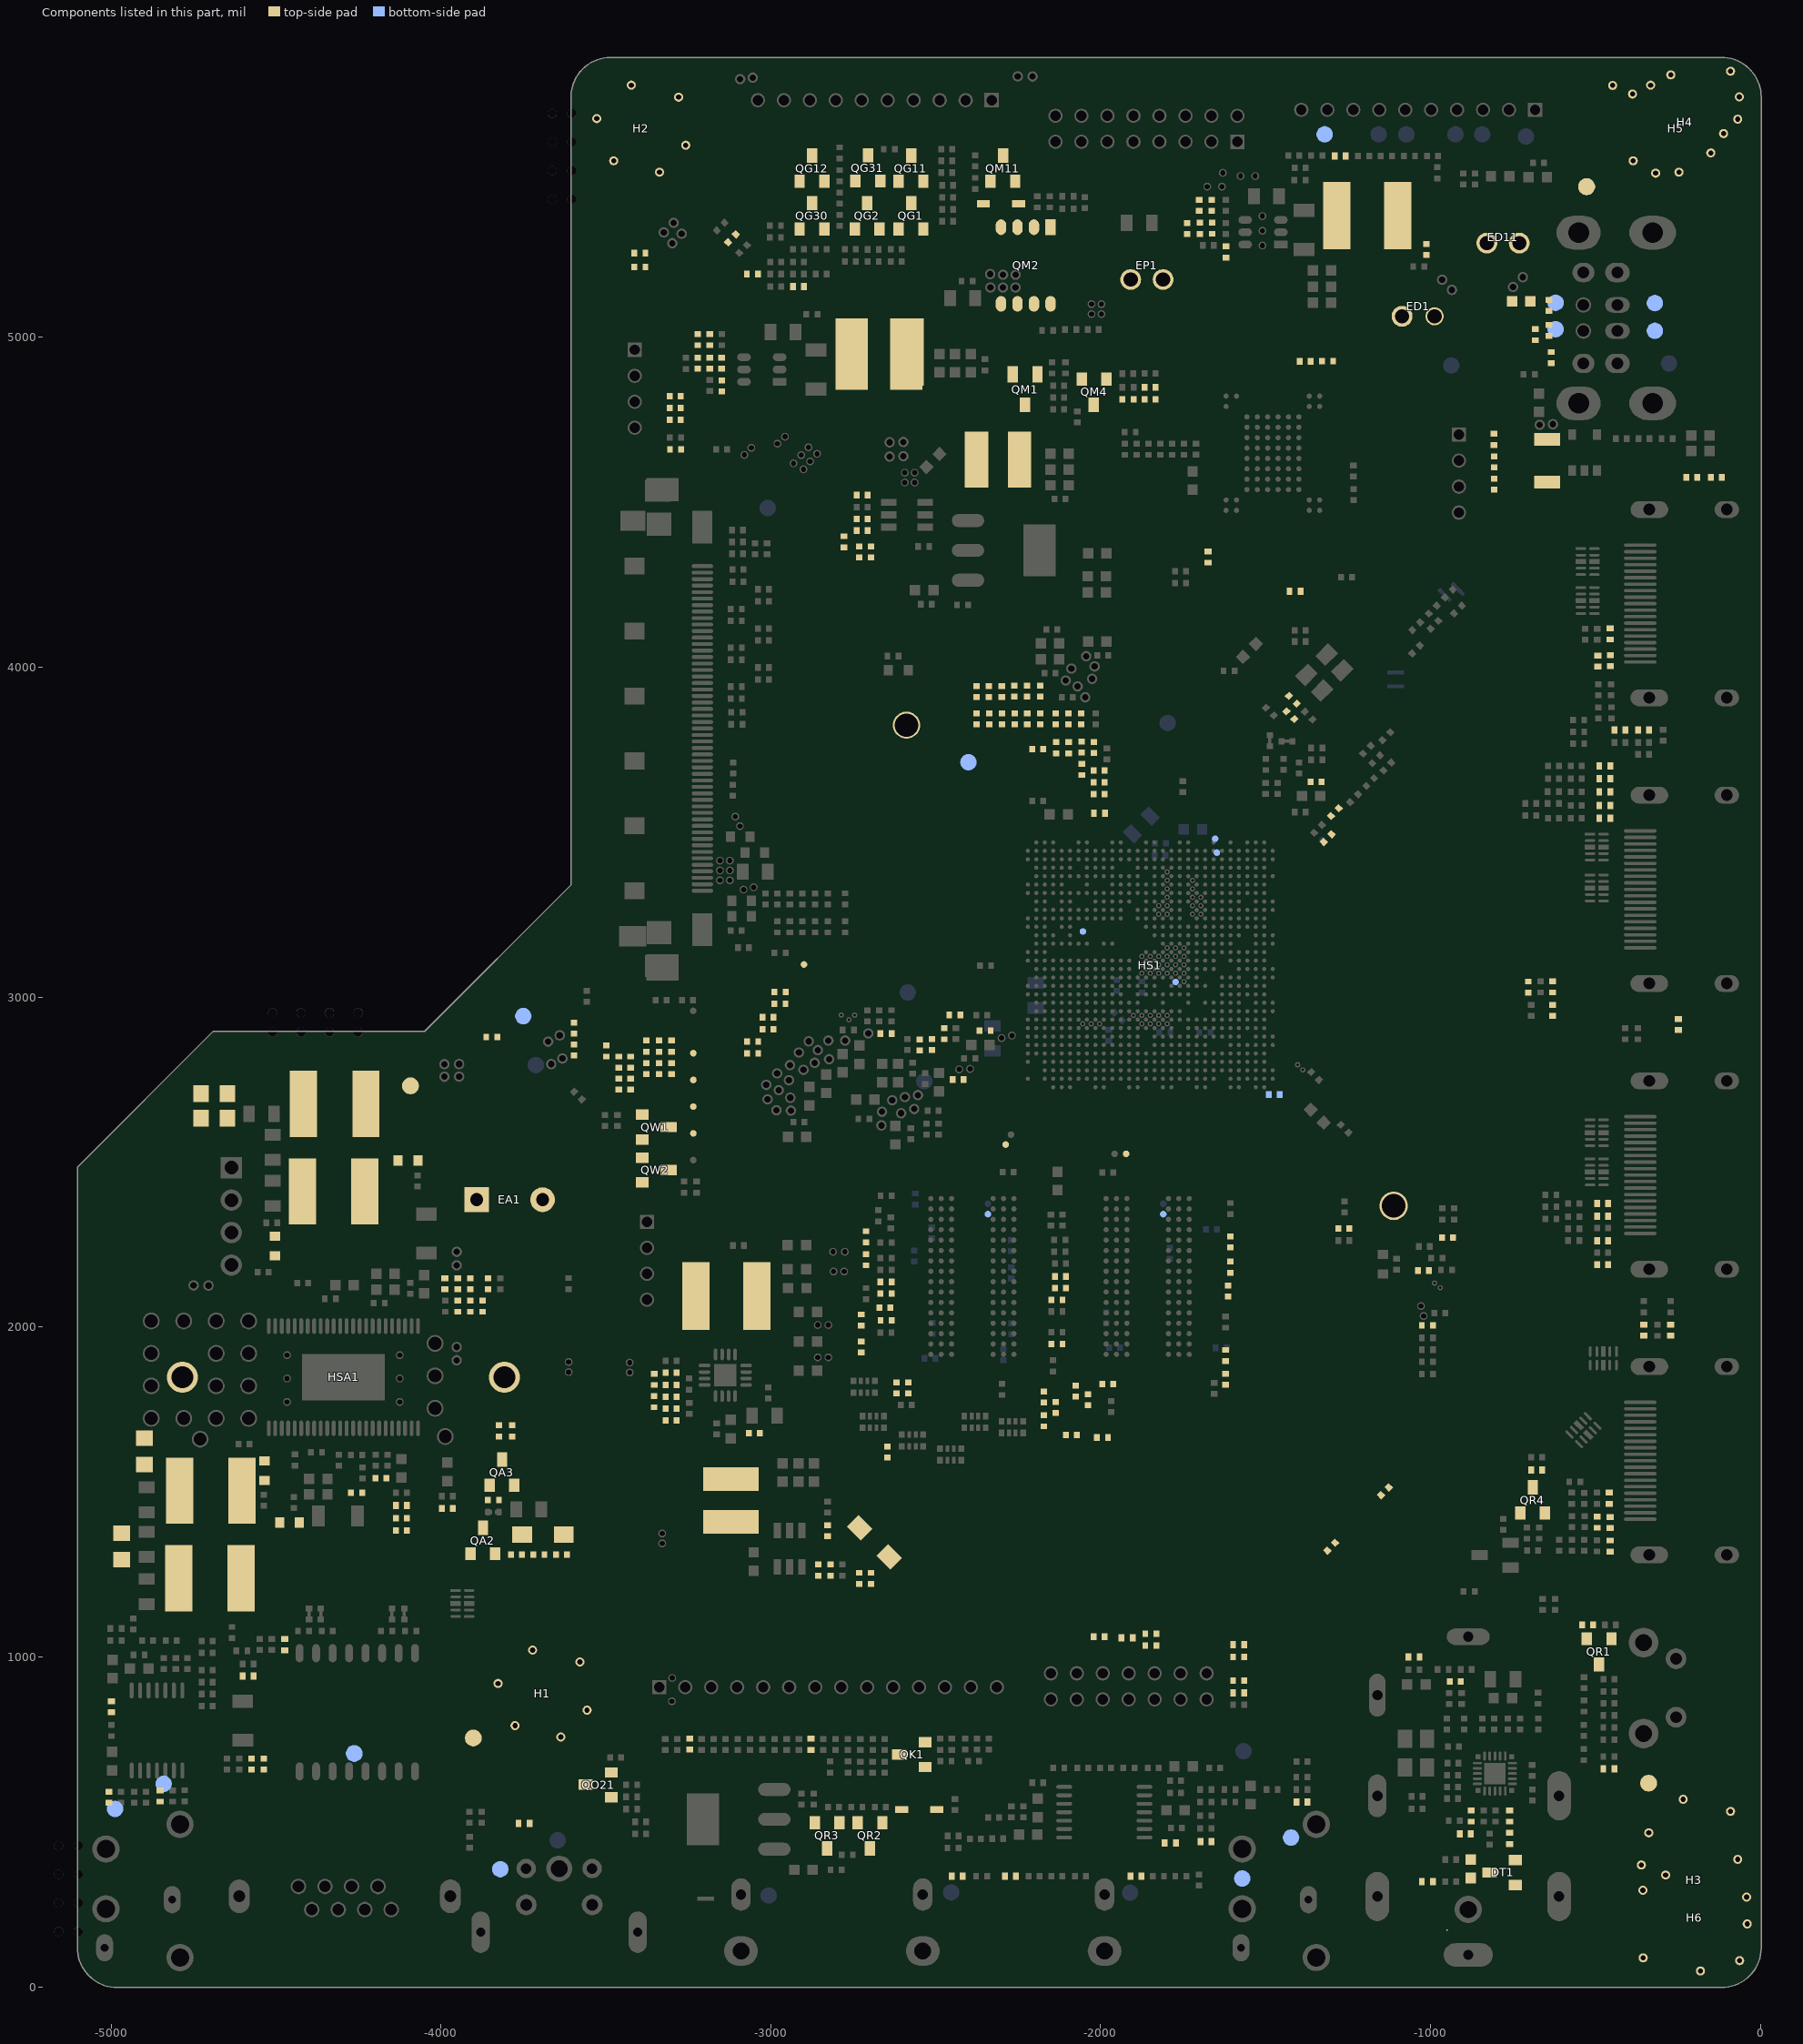
[diagram p0: the components of this part, seen from the top]
# Altium PCB MISC86290.PcbDoc (part 3 of 31)
Units mil, origin at the board's own origin, x right, y up, seen from the top; angles counter-clockwise.
Board outline 5104.71 x 5851.49 mil, 2 copper layers (TopLayer, BottomLayer), stack 61.855 mil thick; 1026 components, 667 nets, 4280 pads, 2294 vias.

## Components (designator, comment, footprint, x,y, rotation, side; value= is the part's Value field where it differs from the comment) (continued)
D41 "NC/SFI0402-240E-2R5PP-LF" DIODE-S0402 -630,2960 r90 top
DA1 "NC/AVLC18S02003" DIODE-S0402 -1582,891 r0 top
DA2 "NC/AVLC18S02003" DIODE-S0402 -1582,1037 r180 top
DA5 "NC/AVLC18S02003" DIODE-S0402 -1920,1058 r0 top
DA6 "NC/AVLC18S02003" DIODE-S0402 -2005,1061 r180 top
DA9 "Switching diode,DIO SW S,200mA,75V,MiniMELF,SMD,LL4148,FORMOSA" DIODE-S0805 -3691,1371 r180 top
DBS7 "DOLBY PLUS" "DOLBY PLUS-SILK" -1080.5,2556.5 r90 bottom
DD2 "Zener diode,DIO ZEN,5.6V,500mW,SOD-80,SMD,BZV55C5V6,GOOD-ARK" DIODE-S0805 -2686,1347 r315 top
DE1 "NC/AIES12U020R2" DIODE-S0402 -4584.6,941.4 r0 top
DE2 "NC/AIES12U020R2" DIODE-S0402 -4473.96,1036.98 r270 top
DF5 "NC/NC/AIES12U020R2" DIODE-S0402 -641.25,5021.27 r90 top
DF6 "NC/NC/AIES12U020R2" DIODE-S0402 -641.25,5096.73 r270 top
DG1 "NC/SFI0402-240E-2R5PP-LF" DIODE-S0402 -2916,5154 r180 top
DG11 "NC/SFI0402-240E-2R5PP-LF" DIODE-S0402 -3056,5192 r0 top
DH1 "NC/TVS diode,DIO ESD,0.5pF,25V,0402 DFN,SMD,AZ5325-01F.R7G,Amazing" DIODE-S0402 -354,3810 r180 top
DH2 "NC/TVS diode,DIO ESD,0.5pF,25V,0402 DFN,SMD,AZ5325-01F.R7G,Amazing" DIODE-S0402 -426,3810 r180 top
DH3 "NC/TVS diode,DIO ESD,0.5pF,25V,0402 DFN,SMD,AZ5325-01F.R7G,Amazing" DIODE-S0402 -455,4019.73 r90 top
DH4 "NC/TVS diode,DIO ESD,0.5pF,25V,0402 DFN,SMD,AZ5325-01F.R7G,Amazing" DIODE-S0402 -493,4019 r90 top
DH5 "NC/TVS diode,DIO ESD,0.5pF,25V,0402 DFN,SMD,AZ5325-01F.R7G,Amazing" DIODE-S0402 -456,4101 r90 top
DH11 "NC/TVS diode,DIO ESD,0.5pF,25V,0402 DFN,SMD,AZ5325-01F.R7G,Amazing" DIODE-S0402 -472,3701 r0 top
DH12 "NC/TVS diode,DIO ESD,0.5pF,25V,0402 DFN,SMD,AZ5325-01F.R7G,Amazing" DIODE-S0402 -472,3662 r0 top
DH13 "NC/TVS diode,DIO ESD,0.5pF,25V,0402 DFN,SMD,AZ5325-01F.R7G,Amazing" DIODE-S0402 -472,3622 r0 top
DH14 "NC/TVS diode,DIO ESD,0.5pF,25V,0402 DFN,SMD,AZ5325-01F.R7G,Amazing" DIODE-S0402 -472,3581 r0 top
DH15 "NC/TVS diode,DIO ESD,0.5pF,25V,0402 DFN,SMD,AZ5325-01F.R7G,Amazing" DIODE-S0402 -472,3542 r0 top
DH21 "NC/TVS diode,DIO ESD,0.5pF,25V,0402 DFN,SMD,AZ5325-01F.R7G,Amazing" DIODE-S0402 -478,2189 r0 top
DH22 "NC/TVS diode,DIO ESD,0.5pF,25V,0402 DFN,SMD,AZ5325-01F.R7G,Amazing" DIODE-S0402 -478,2261 r0 top
DH23 "NC/TVS diode,DIO ESD,0.5pF,25V,0402 DFN,SMD,AZ5325-01F.R7G,Amazing" DIODE-S0402 -478,2336 r0 top
DH24 "NC/TVS diode,DIO ESD,0.5pF,25V,0402 DFN,SMD,AZ5325-01F.R7G,Amazing" DIODE-S0402 -478,2374 r0 top
DH31 "NC/TVS diode,DIO ESD,0.5pF,25V,0402 DFN,SMD,AZ5325-01F.R7G,Amazing" DIODE-S0402 -456,1407 r270 top
DH32 "NC/TVS diode,DIO ESD,0.5pF,25V,0402 DFN,SMD,AZ5325-01F.R7G,Amazing" DIODE-S0402 -456,1336 r270 top
DH33 "NC/TVS diode,DIO ESD,0.5pF,25V,0402 DFN,SMD,AZ5325-01F.R7G,Amazing" DIODE-S0402 -495,1408 r90 top
DH34 "NC/TVS diode,DIO ESD,0.5pF,25V,0402 DFN,SMD,AZ5325-01F.R7G,Amazing" DIODE-S0402 -458,1481 r90 top
DH35 "NC/TVS diode,DIO ESD,0.5pF,25V,0402 DFN,SMD,AZ5325-01F.R7G,Amazing" DIODE-S0402 -353.27,1990.5 r90 top
DH36 "NC/TVS diode,DIO ESD,0.5pF,25V,0402 DFN,SMD,AZ5325-01F.R7G,Amazing" DIODE-S0402 -272,1990.5 r90 top
DH37 "NC/TVS diode,DIO ESD,0.5pF,25V,0402 DFN,SMD,AZ5325-01F.R7G,Amazing" DIODE-S0402 -248.64,2917.23 r270 top
DI1 "NC/TVS diode,DIO ESD,3pF,58V,0402,SMD,SDV1005H260C030YPTF,Sunlord" DIODE-S0402 -2435,335 r0 top
DI2 "NC/TVS diode,DIO ESD,3pF,58V,0402,SMD,SDV1005H260C030YPTF,Sunlord" DIODE-S0402 -2274,335 r0 top
DI3 "NC/TVS diode,DIO ESD,3pF,58V,0402,SMD,SDV1005H260C030YPTF,Sunlord" DIODE-S0402 -1893,335 r180 top
DK9 "NC/AVLC18S02003" DIODE-S0402 -2878.25,735 r270 top
DK10 "NC/AVLC18S02003" DIODE-S0402 -3245.92,735.99 r270 top
DM0 "TEST" TP -320,5020 r180 bottom
DM1 "TEST" TP -620.95,5024.72 r180 bottom
DM11 "NC/Switching diode,DIO SW S,150mA,75V,SOD-323,SMD,1N4148WS,BLUE ROCKET" DIODE-S-12 -2302.25,5405 r180 top
DO1 "NC/SFI0402-240E-2R5PP-LF" DIODE-S0402 -3748.25,495 r180 top
DO2 "NC/SFI0402-240E-2R5PP-LF" DIODE-S0402 -1022,2171 r0 top
DO11 "NC/NC?" DIODE-S0402 -1390,559.5 r0 top
DO12 "NC/NC?" DIODE-S0402 -1681,440 r0 top
DO31 "NC/NC?" DIODE-S0402 -4851.5,578 r270 top
DO32 "NC/NC?" DIODE-S0402 -5006.75,573.94 r270 top
DP0 "TEST" TP -320,5104 r180 bottom
DP1 "TEST" TP -620.95,5105.12 r180 bottom
DQS0 "TEST" TP-20#1 -1923,2525 r90 top
DQS0# "TEST" TP-20#1 -1958,2525 r90 top
DQS1 "TEST" TP-20#1 -1810.35,2342.13 r90 bottom
DQS1# "TEST" TP-20#1 -1810.35,2373.62 r90 bottom
DQS2 "TEST" TP-20#1 -2288,2553 r90 top
DQS2# "TEST" TP-20#1 -2272,2583 r90 top
DQS3 "TEST" TP-20#1 -2341.85,2342.13 r90 bottom
DQS3# "TEST" TP-20#1 -2341.85,2373.62 r90 bottom
DR1 "NC/TVS diode,DIO ESD,3pF,58V,0402,SMD,SDV1005H260C030YPTF,Sunlord" DIODE-S0402 -678.5,1566.5 r0 top
DR2 "TVS diode,DIO ESD,3pF,58V,0402,SMD,SDV1005H260C030YPTF,Sunlord" DIODE-S0402 -459.5,660.5 r0 top
DR3 "Switching diode,DIO SW S,150mA,75V,SOD-323,SMD,1N4148WS,BLUE ROCKET" DIODE-S-12 -2550,537 r180 top
DR4 "NC/TVS diode,DIO ESD,3pF,58V,0402,SMD,SDV1005H260C030YPTF,Sunlord" DIODE-S0402 -1474,2704.5 r180 bottom
DR5 "NC/TVS diode,DIO ESD,3pF,58V,0402,SMD,SDV1005H260C030YPTF,Sunlord" DIODE-S0402 -2004,3557.11 r180 top
DT1 "Switching diode,DIO SW D2,75V,SOT-23,SMD,KAV99,KEXIN" SO-23 -782.86,346.15 r270 top
DT2 "NC/TVS diode,DIO ESD,3pF,58V,0402,SMD,SDV1005H260C030YPTF,Sunlord" DIODE-S0402 -208,4576 r0 top
DT3 "NC/TVS diode,DIO ESD,3pF,58V,0402,SMD,SDV1005H260C030YPTF,Sunlord" DIODE-S0402 -134,4576 r180 top
DU1 "NC/AIES12U020R2" DIODE-S0402 -634,4939 r90 top
DU2 "NC/AIES12U020R2" DIODE-S0402 -682.3,5008.37 r270 top
DVDD_DDR "TEST" TP-20#1 -1773,3046.11 r90 bottom
DW1 "NC/AIES12U020R2" DIODE-S0402 -1274,5550 r180 top
DW2 "NC/AIES12U020R2" DIODE-S0402 -1411,4230 r0 top
EA1 "Aluminium electrolytic capacitor,CAP AL,16V,470uF,±20%,KM,P,5.0mm,10×12.5,DIP,TP,Samxon" EC(10*13)-V-5.0-1 -3792,2386 r0 top
ED1 "Aluminium electrolytic capacitor,CAP AL,10V,470uF,±20%,PKZH,P,2.5mm,6.3×11,DIP,TP,Koshin" EC(6.3*11)-V-2.5#1 -1037.21,5064 r0 top
ED11 "Aluminium electrolytic capacitor,CAP AL,10V,470uF,±20%,PKZH,P,2.5mm,6.3×11,DIP,TP,Koshin" EC(6.3*11)-V-2.5#2 -780.27,5286 r0 top
EJ_TCK "TEST" TP-20#1 -3235,2587 r0 top
EJ_TDI "TEST" TP-20#1 -3235,2668 r0 top
EJ_TDO "TEST" TP-20#1 -3235,2749 r0 top
EJ_TMS "TEST" TP-20#1 -3235,2830 r0 top
EP1 "Aluminium electrolytic capacitor,CAP AL,16V,220uF,±20%,LD,KF,P,2.5mm,6.3×11,DIP,TP,CapXon" EC(6.3*11)-V-2.5#3 -1860,5175.5 r0 top
FT1 "Ferrite bead,BEAD,120ohm,0402,500mA,SMD,TP,GZ1005U121CTF,Sunlord" L0402 -1050,1000 r0 top
FU1 "NC/Resettable fuse,FUSE PTC,1.1A,6V,1206,SMD,TP,TLC" FUSE1.1A-S -647,4626 r270 top
H1 "Location hole" ASSE3.5C-3#1 -3685.04,885.83 r0 top locked
H2 "Location hole" ASSE3.5C-3#2 -3385.83,5629.92 r0 top locked
H3 "Location hole" ASSE3.5C-3#3 -196.85,433.07 r0 top locked
H4 "Location hole" ASSE3.5C-3#4 -196.85,5708.66 r0 top locked
H5 "Location hole" ASSE3.5C-3#5 -295.28,5629.92 r0 top locked
H6 "Location hole" ASSE5.0C-3 -196.85,196.85 r0 top locked
HOST_WAKE_WL "TEST" TP -1321.08,5615.53 r180 bottom locked
HP_DET "TEST" TP -3750.5,2942.5 r180 bottom
HP_OUT_L "TEST" TP -1570.87,328 r90 bottom
HP_OUT_R "TEST" TP -1423,452 r90 bottom
HS1 "Heat sink,AL6063-T5,55.0×55.0×10.0mm,black,anodized,fin type,LHD" HS(55*55*10) -1849.72,3098.03 r270 top locked
HSA1 "NC/Heat sink,27.5×10.0×10.0mm,AL6063-T5,black,anodized,fin type,WT" HS(27*10*10)-1 -4295.75,1847.75 r90 top locked
I2S_IN_MCK "TEST" TP-20#1 -2899.5,3099 r90 top
LA1 "Power inductor,Power Inductor,15uH,±20%,2.10A,DR6.0×4.5,SMD,MPIT6045-150M-LF,Microgate" L(6.0*4.5)-S#1 -4700.74,1238 r180 top
LA2 "Power inductor,Power Inductor,15uH,±20%,2.10A,DR6.0×4.5,SMD,MPIT6045-150M-LF,Microgate" L(6.0*4.5)-S#1 -4697.39,1503.52 r180 top
LA3 "Power inductor,Power Inductor,15uH,±20%,2.10A,DR6.0×4.5,SMD,MPIT6045-150M-LF,Microgate" L(6.0*4.5)-S#1 -4325,2411 r0 top
LA4 "Power inductor,Power Inductor,15uH,±20%,2.10A,DR6.0×4.5,SMD,MPIT6045-150M-LF,Microgate" L(6.0*4.5)-S#1 -4322,2676.38 r180 top
LA10 "0ohm-0402-±5%-1/16W" L0402 -3988,2131 r270 top
LA12 "0ohm-0402-±5%-1/16W" L0402 -4120,1459 r0 top
LD1 "NC/Power inductor,Power Inductor,4.7uH,±20%,3.3A,DR6.0×4.5,SMD,SWPA6045S4R7MT,Sunlord" L(6.0*4.5)-S#2 -1192.25,5369 r0 top
LD2 "Power inductor,Power Inductor,4.7uH,±20%,2.8A,0.32×1P,DR5.8×4.5,SMD,PIO54-4R7MTP02,FH" L(5.8*4.5)-S -2672.12,4949.21 r0 top
LD3 "NC/Power inductor,Power Inductor,4.7uH,±20%,3.8A,DR6.0×4.5,SMD,MPIT6045-4R7M-LF,Microgate" L(6.0*4.5)-S#2 -2670,4955.5 r0 top
LD4 "Power inductor,Power Inductor,4.7uH,±20%,3.3A,DR6.0×4.5,SMD,PRS6045-4R7MTP02,FH" L(6.0*4.5)-S#2 -1192.25,5369 r0 top
LD21 "Power inductor,Power Inductor,2.2uH,±20%,2A,0.28×1P,DR4.5×3.2,SMD,PIO43-2R2MTP02,FH" L(4.5*3.5)-S -3121,1474 r90 top
LD31 "Power inductor,Power Inductor,2.2μH,±30%,4.6A,6045,SMT,PRS6045-2R2NTP02,FH" L(6.0*4.5)-S#2 -3134.25,2094 r0 top
LD51 "Power inductor,Power Inductor,2.2uH,±20%,2A,0.28×1P,DR4.5×3.2,SMD,PIO43-2R2MTP02,FH" L(4.5*3.5)-S -2311.2,4629.43 r0 top
LF1 "0ohm-0402-±5%-1/16W" L0402 -1675,4334 r270 top
LINEOUT_L "TEST" TP -4988,539 r90 bottom
LINEOUT_R "TEST" TP -4840.5,615 r90 bottom
LO1 "0ohm-0402-±5%-1/16W" R0402 -1347.27,3653 r0 top
LO2 "Ferrite bead,BEAD,120ohm,0402,500mA,SMD,TP,GZ1005U121CTF,Sunlord" L0402 -1789,436 r180 top
LO3 "Ferrite bead,BEAD,120ohm,0402,500mA,SMD,TP,GZ1005U121CTF,Sunlord" L0402 -4999,849 r90 top
LT3 "0ohm-0402-±5%-1/16W" L0402 -894.9,463.14 r180 top
LT4 "SDCL1005CR33JTDF" L0402 -1009.7,318.3 r180 top
LT5 "SDCL1005CR33JTDF" L0402 -876.89,517.36 r270 top
LT6 "SDCL1005CR33JTDF" L0402 -759.9,517.37 r270 top
LT7 "0ohm-0402-±5%-1/16W" L0402 -760.22,449.51 r270 top
LT9 "NC/Multilayer inductor,HF Inductor,180nH,±5%,0603,SMD,SDCL1608CR18JTDF,Sunlord" L0603 -877.7,357.3 r90 top
LT10 "NC/" R0402 -924.82,925.61 r0 top
LU11 "HCB1608KF-121T20(120ohm-2000mA)" L0603 -725,5110 r0 top
M1 "MARK" MARK -3902,754 r0 top
M2 "MARK" MARK -527,5457 r0 top
M3 "MARK" MARK -339,617 r0 top
M4 "MARK" MARK -4092.5,2731 r0 top
M5 "MARK" MARK -527,5457 r180 bottom
M6 "MARK" MARK -4263,707 r180 bottom
MAC "MAC" Barcode -2576,4726 r180 bottom
Manufacture_Info "Manufacture_Info" Manufacture_Info -1486,4578 r270 top
MCP_TEST "TEST" TP-20#1 -2054,3199 r180 bottom
MOD_1V2 "TEST" TP -2401,3712.11 r90 bottom
NC/ESD "NC/ESD" ESD -926.56,194.83 r225 top
OPTICAL "TEST" TP -3820.25,356.18 r90 bottom
P1(用于U1上) "Thermal grease,0.05g,Other,white,NULL" PCB_TIME -386,-235 r180 top
PM_RX "TEST" TP-20#2 -1648,3438 r180 bottom
PM_TX "TEST" TP-20#2 -1653,3480 r180 bottom
QA2 "General-purpose transistor,Dynatron,PNP,0.2A,40V,30-100,SOT-23,MMBT3906-(100-300),BLUE ROCKET" SOT-23 -3873,1353 r180 top
QA3 "General-purpose transistor,Dynatron,NPN,0.2A,40V,30-300,SOT-23,MMBT3904(f≥350MHz),BLUE ROCKET" SOT-23 -3815,1560 r180 top
QG1 "NC/General-purpose transistor,Dynatron,NPN,0.2A,40V,60-300,SOT-23,KMBT3904,KEXIN" SOT-23 -2575.25,5369 r180 top
QG2 "NC/General-purpose transistor,Dynatron,NPN,0.2A,40V,60-300,SOT-23,KMBT3904,KEXIN" SOT-23 -2708,5369 r180 top
QG11 "NC/General-purpose transistor,Dynatron,NPN,0.2A,40V,60-300,SOT-23,KMBT3904,KEXIN" SOT-23 -2575.25,5513.12 r180 top
QG12 "NC/General-purpose transistor,Dynatron,NPN,0.2A,40V,60-300,SOT-23,KMBT3904,KEXIN" SOT-23 -2875.31,5513.12 r180 top
QG30 "NC/General-purpose transistor,Dynatron,NPN,0.2A,40V,60-300,SOT-23,KMBT3904,KEXIN" SOT-23 -2875.31,5369 r180 top
QG31 "NC/General-purpose transistor,Dynatron,NPN,0.2A,40V,60-300,SOT-23,KMBT3904,KEXIN" SOT-23 -2706,5514 r180 top
QK1 "General-purpose transistor,Dynatron,NPN,0.2A,40V,60-300,SOT-23,KMBT3904,KEXIN" SOT-23 -2572.5,703.5 r270 top
QM1 "MOSFET,PMOS,-4.2A,-30V,0.052ohm@ID=-4.2A@VGS=-10V,SOT23-3,AO3401,BLUE ROCKET" SOT-23-1 -2229,4841 r0 top
QM2 "MOSFET,PMOS,-5.7A,-30V,0.07ohm@ID=-4.4A@VGS=-4.5V,SOP-8,KO4459,KEXIN" SO-8 -2227.25,5218 r270 top locked
QM4 "General-purpose transistor,Dynatron,NPN,0.2A,40V,60-300,SOT-23,KMBT3904,KEXIN" SOT-23 -2020.25,4834 r0 top
QM11 "General-purpose transistor,Dynatron,NPN,0.2A,40V,60-300,SOT-23,KMBT3904,KEXIN" SOT-23 -2296.75,5513.13 r180 top
QO21 "General-purpose transistor,Dynatron,NPN,0.2A,40V,60-300,SOT-23,KMBT3904,KEXIN" SOT-23 -3523.5,612 r270 top
QR1 "KMBT3906" SOT-23 -489,1015 r0 top
QR2 "KMBT3906" SOT-23 -2699.25,457 r0 top
QR3 "General-purpose transistor,Dynatron,NPN,0.2A,40V,60-300,SOT-23,KMBT3904,KEXIN" SOT-23 -2829.25,457 r0 top
QR4 "General-purpose transistor,Dynatron,NPN,0.2A,40V,60-300,SOT-23,KMBT3904,KEXIN" SOT-23 -690.6,1476 r180 top
QW1 "NC/MOSFET,NMOS,0.3A,60V,3.3ohm@ID=0.3A@VGS=4.5V,SOT-23,ME2N7002E,MATSUKI" SOT-23-7 -3350,2606 r270 top
QW2 "NC/MOSFET,NMOS,0.3A,60V,3.3ohm@ID=0.3A@VGS=4.5V,SOT-23,ME2N7002E,MATSUKI" SOT-23-7 -3350,2476 r270 top
R1 "0ohm-0402-±5%-1/16W" R0402 -2650.73,2889.5 r0 top
R3 "0ohm-0402-±5%-1/16W" R0402 -1009.73,2004.84 r0 top
R4 "Thick-film resistor,RES,1/16W,4.7Kohm,±5%,0402,SMD" R0402 -2136,3844 r90 top
R5 "NC/Thick-film resistor,RES,1/16W,4.7Kohm,±5%,0402,SMD" R0402 -2098,3844 r90 top
R6 "NC/Thick-film resistor,RES,1/16W,4.7Kohm,±5%,0402,SMD" R0402 -2183.75,3927.72 r90 top
R7 "NC/Thick-film resistor,RES,1/16W,4.7Kohm,±5%,0402,SMD" R0402 -2005,3651 r0 top
R8 "NC/Thick-film resistor,RES,1/16W,4.7Kohm,±5%,0402,SMD" R0402 -2191,3752 r0 top
R9 "Thick-film resistor,RES,1/16W,4.7Kohm,±5%,0402,SMD" R0402 -2135,3756 r270 top
R10 "Thick-film resistor,RES,1/16W,4.7Kohm,±5%,0402,SMD" R0402 -2183.75,3843.79 r270 top
R11 "Thick-film resistor,RES,1/16W,4.7Kohm,±5%,0402,SMD" R0402 -2005,3615 r180 top
R12 "NC/Thick-film resistor,RES,1/16W,4.7Kohm,±5%,0402,SMD" R0402 -2261.75,3927.5 r90 top
R13 "NC/Thick-film resistor,RES,1/16W,4.7Kohm,±5%,0402,SMD" R0402 -2376.75,3926.5 r90 top
R14 "NC/Thick-film resistor,RES,1/16W,4.7Kohm,±5%,0402,SMD" R0402 -2223.75,3927.5 r90 top
R15 "NC/Thick-film resistor,RES,1/16W,4.7Kohm,±5%,0402,SMD" R0402 -2299.75,3926.5 r90 top
R16 "NC/Thick-film resistor,RES,1/16W,4.7Kohm,±5%,0402,SMD" R0402 -2059,3844 r90 top
R17 "NC/Thick-film resistor,RES,1/16W,4.7Kohm,±5%,0402,SMD" R0402 -2021,3757 r90 top
R18 "Thick-film resistor,RES,1/16W,4.7Kohm,±5%,0402,SMD" R0402 -2338.75,3926.5 r90 top
R19 "Thick-film resistor,RES,1/16W,4.7Kohm,±5%,0402,SMD" R0402 -2005,3687 r0 top
R20 "Thick-film resistor,RES,1/16W,4.7Kohm,±5%,0402,SMD" R0402 -2260.75,3843.57 r270 top
R21 "Thick-film resistor,RES,1/16W,4.7Kohm,±5%,0402,SMD" R0402 -2376.75,3843.57 r270 top
R22 "Thick-film resistor,RES,1/16W,4.7Kohm,±5%,0402,SMD" R0402 -2222.75,3843.57 r270 top
R23 "Thick-film resistor,RES,1/16W,4.7Kohm,±5%,0402,SMD" R0402 -2298.75,3843.57 r270 top
R24 "Thick-film resistor,RES,1/16W,4.7Kohm,±5%,0402,SMD" R0402 -2097,3756 r270 top
R25 "Thick-film resistor,RES,1/16W,4.7Kohm,±5%,0402,SMD" R0402 -2058,3758 r270 top
R26 "NC/Thick-film resistor,RES,1/16W,4.7Kohm,±5%,0402,SMD" R0402 -2337.75,3843.57 r270 top
R27 "NC/Thick-film resistor,RES,1/16W,4.7Kohm,±5%,0402,SMD" R0402 -2057,3690 r270 top
R30 "4K7ohm-0402-±5%-1/16W" R0402 -3289.5,4750.37 r0 top
R31 "4K7ohm-0402-±5%-1/16W" R0402 -3289.5,4786.37 r0 top
R39 "Thick-film resistor,RES,1/16W,68ohm,±5%,0402,SMD" R0402 -1290,3561 r225 top
R41 "Thick-film resistor,RES,1/16W,75ohm,±5%,0402,SMD" R0402 -1312,3482 r225 top
R42 "1Mohm-0402-±5%-1/16W" R0402 -1417.47,3901.53 r315 top
R44 "Thick-film resistor,RES,1/16W,1Kohm,±5%,0402,SMD" R0402 -2548.87,2854.84 r270 top
R45 "Thick-film resistor,RES,1/16W,10Kohm,±5%,0402,SMD" R0402 -2442.46,2946.03 r0 top
R46 "Thick-film resistor,RES,1/16W,1Kohm,±1%,0402,SMD" R0402 -2511.84,2856.32 r270 top
R47 "Thick-film resistor,RES,1/16W,1Kohm,±1%,0402,SMD" R0402 -2474.76,2888.9 r90 top
R48 "Thick-film resistor,RES,1/16W,240ohm,±1%,0402,SMD" R0402 -2432.46,2750.03 r0 top
R49 "Thick-film resistor,RES,1/16W,240ohm,±1%,0402,SMD" R0402 -2350.46,2898.03 r0 top
R50 "Thick-film resistor,RES,1/16W,22ohm,±5%,0402,SMD" R0402 -2122.05,2153.15 r180 top
R51 "Thick-film resistor,RES,1/16W,22ohm,±5%,0402,SMD" R0402 -2122.05,2117.72 r180 top
R52 "Thick-film resistor,RES,1/16W,22ohm,±5%,0402,SMD" R0402 -1606.61,2181.38 r270 top
R53 "Thick-film resistor,RES,1/16W,22ohm,±5%,0402,SMD" R0402 -2136.3,1755.67 r270 top
R54 "Thick-film resistor,RES,1/16W,75ohm,±5%,0402,SMD" R0402 -2038.7,1779.8 r270 top
R55 "Thick-film resistor,RES,1/16W,75ohm,±5%,0402,SMD" R0402 -2076.1,1805.39 r270 top
R56 "Thick-film resistor,RES,1/16W,22ohm,±5%,0402,SMD" R0402 -2089.21,1672.83 r180 top
R57 "Thick-film resistor,RES,1/16W,22ohm,±5%,0402,SMD" R0402 -2725.97,1939.76 r90 top
R58 "Thick-film resistor,RES,1/16W,75ohm,±5%,0402,SMD" R0402 -2618.69,1815.24 r90 top
R59 "Thick-film resistor,RES,1/16W,75ohm,±5%,0402,SMD" R0402 -1994.72,1664.96 r180 top
R60 "Thick-film resistor,RES,1/16W,75ohm,±5%,0402,SMD" R0402 -2653.99,2058.66 r0 top
R61 "Thick-film resistor,RES,1/16W,75ohm,±5%,0402,SMD" R0402 -2646.25,1620.98 r90 top
R62 "Thick-film resistor,RES,1/16W,10Kohm,±5%,0402,SMD" R0402 -1606.61,2258.15 r270 top
R63 "Thick-film resistor,RES,1/16W,10Kohm,±5%,0402,SMD" R0402 -1978.66,1826.69 r180 top
R64 "Thick-film resistor,RES,1/16W,240ohm,±1%,0402,SMD" R0402 -1613.5,2109.17 r90 top
R65 "Thick-film resistor,RES,1/16W,620ohm,±1%,0402,SMD" R0402 -2172.56,1715.47 r90 top
R66 "Thick-film resistor,RES,1/16W,10Kohm,±1%,0402,SMD" R0402 -1621.38,1841.46 r270 top
R67 "Thick-film resistor,RES,1/16W,10Kohm,±1%,0402,SMD" R0402 -1621.38,1913.66 r270 top
R72 "100ohm-0402-±5%-1/16W" R0402 -1312,4928 r0 top
R73 "100ohm-0402-±5%-1/16W" R0402 -1380,4927.5 r0 top
R100 "Thick-film resistor,RES,1/16W,240ohm,±1%,0402,SMD" R0402 -2132.52,2082.28 r180 top
R101 "Thick-film resistor,RES,1/16W,620ohm,±1%,0402,SMD" R0402 -2650.63,2019.83 r180 top
R102 "Thick-film resistor,RES,1/16W,620ohm,±1%,0402,SMD" R0402 -2725.97,2021.3 r90 top
R103 "Thick-film resistor,RES,1/16W,10Kohm,±1%,0402,SMD" R0402 -2711.26,2273.63 r90 top
R104 "Thick-film resistor,RES,1/16W,10Kohm,±1%,0402,SMD" R0402 -2711.21,2203.66 r90 top
R105 "Thick-film resistor,RES,1/16W,56ohm,±1%,0402,SMD" R0402 -2650.85,2100.98 r0 top
R106 "Thick-film resistor,RES,1/16W,56ohm,±1%,0402,SMD" R0402 -2650.85,2136.42 r0 top
R107 "Thick-film resistor,RES,1/16W,10Kohm,±5%,0402,SMD" R0402 -2583.26,1815.24 r90 top
R108 "Thick-film resistor,RES,1/16W,10Kohm,±5%,0402,SMD" R0402 -2132.52,1948.43 r180 top
R118 "Thick-film resistor,RES,1/16W,620ohm,±1%,0402,SMD" R0402 -2172.56,1787.68 r90 top
R120 "Thick-film resistor,RES,1/16W,1Kohm,±5%,0402,SMD" R0402 -2732.16,1238 r270 top
R121 "Thick-film resistor,RES,1/16W,10Kohm,±5%,0402,SMD" R0402 -2696.16,1238 r90 top
R122 "Thick-film resistor,RES,1/16W,2.2Kohm,±5%,0402,SMD" R0402 -3949,2131 r90 top
R123 "Thick-film resistor,RES,1/16W,1Kohm,±5%,0402,SMD" R0402 -1263.27,2299 r180 top
R124 "Thick-film resistor,RES,1/16W,2.2Kohm,±5%,0402,SMD" R0402 -3911,2131 r90 top
R125 "Thick-film resistor,RES,1/16W,33ohm,±5%,0402,SMD" R0402 -3397,5255.5 r0 top
R126 "Thick-film resistor,RES,1/16W,33ohm,±5%,0402,SMD" R0402 -3377,2783.5 r90 top
R127 "Thick-film resistor,RES,1/16W,33ohm,±5%,0402,SMD" R0402 -3377,2851.5 r270 top
R128 "Thick-film resistor,RES,1/16W,33ohm,±5%,0402,SMD" R0402 -3499,2836.5 r90 top
R129 "Thick-film resistor,RES,1/16W,33ohm,±5%,0402,SMD" R0402 -3118,5300.5 r45 top
R130 "0ohm-0402-±5%-1/16W" R0402 -3397,5214 r0 top
R135 "0ohm-0402-±5%-1/16W" R0402 -1301,1334 r225 top
R136 "0ohm-0402-±5%-1/16W" R0402 -1138.5,1502 r225 top
R137 "0ohm-0402-±5%-1/16W" R0402 -808,4691 r90 top
R138 "4K7ohm-0402-±5%-1/16W" R0402 -807,4555 r90 top
R139 "4K7ohm-0402-±5%-1/16W" R0402 -807,4623 r270 top
R140 "100ohm-0402-±5%-1/16W" R0402 -630,3031 r270 top
R141 "100ohm-0402-±5%-1/16W" R0402 -704,3030.5 r270 top
R143 "NC/4K7ohm-0402-±5%-1/16W" R0402 -3597,2906 r90 top
R144 "4K7ohm-0402-±5%-1/16W" R0402 -3461,2736.1 r270 top
R145 "4K7ohm-0402-±5%-1/16W" R0402 -3425,2736 r270 top
R146 "33ohm-0402-±5%-1/16W" R0402 -3339,2851.5 r270 top
R147 "33ohm-0402-±5%-1/16W" R0402 -3461,2803 r270 top
R148 "33ohm-0402-±5%-1/16W" R0402 -3339,2783.5 r270 top
R149 "33ohm-0402-±5%-1/16W" R0402 -3425,2803 r270 top
R150 "33ohm-0402-±5%-1/16W" R0402 -3597,2840 r90 top
R151 "4K7ohm-0402-±5%-1/16W" R0402 -948.77,2271.3 r0 top
R152 "4K7ohm-0402-±5%-1/16W" R0402 -1013,5267 r90 top
R153 "4K7ohm-0402-±5%-1/16W" R0402 -523.73,1097 r0 top
R171 "0ohm-0402-±5%-1/16W" R0402 -3289.5,4822.37 r0 top
R200 "100ohm-0402-±5%-1/16W" R0402 -2972.23,2979.5 r0 top
R201 "100ohm-0402-±5%-1/16W" R0402 -2972,3016 r0 top
R202 "100ohm-0402-±5%-1/16W" R0402 -3008.77,2939 r0 top
R203 "100ohm-0402-±5%-1/16W" R0402 -3008.77,2902.5 r0 top
R204 "100ohm-0402-±5%-1/16W" R0402 -3054.98,2865.52 r0 top
R205 "100ohm-0402-±5%-1/16W" R0402 -3054.98,2829.02 r0 top
R206 "4K7ohm-0402-±5%-1/16W" R0402 -3301,2851.5 r270 top
R207 "4K7ohm-0402-±5%-1/16W" R0402 -3301,2783.5 r90 top
R208 "0ohm-0402-±5%-1/16W" R0402 -1424.98,3854.68 r315 top
RA1 "22ohm-0402-±5%-1/16W" R0402 -1848,1070 r180 top
RA2 "22ohm-0402-±5%-1/16W" R0402 -1848,1034 r180 top
RA3 "22ohm-0402-±5%-1/16W" R0402 -1582,1000 r180 top
RA4 "22ohm-0402-±5%-1/16W" R0402 -1582,928 r0 top
RA5 "10Kohm-0402-±5%-1/16W" R0402 -4120,1420 r0 top
RA6 "470ohm-0402-±5%-1/16W" R0402 -4181.75,1541.81 r0 top
RA7 "NC/10Kohm-0402-±5%-1/16W" R0402 -4120,1383 r180 top
RA8 "470ohm-0402-±5%-1/16W" R0402 -4255.75,1497.81 r0 top
RA9 "100ohm-0402-±5%-1/16W" R0402 -3824,1685 r90 top
RA11 "4K7ohm-0402-±5%-1/16W" R0402 -3874,2063 r270 top
RA12 "100ohm-0402-±5%-1/16W" R0402 -3857.35,2131.03 r90 top
RA14 "100ohm-0402-±5%-1/16W" R0402 -3949,2063 r270 top
RA15 "18Kohm-0402-±1%-1/16W" R0402 -3981,1450 r0 top
RA16 "NC/18ohm-0603-±5%-1/10W" R0603 -4459.39,1407.52 r0 top
RA17 "NC/18ohm-0603-±5%-1/10W" R0603 -4535.39,1564.52 r270 top
RA18 "NC/18ohm-0603-±5%-1/10W" R0603 -4503.77,2245.01 r90 top
RA19 "NC/18ohm-0603-±5%-1/10W" R0603 -4100,2505 r0 top
RA20 "4K7ohm-0402-±5%-1/16W" R0402 -3784,1685 r270 top
RA21 "100ohm-0402-±5%-1/16W" R0402 -3911,2063 r90 top
RA22 "8K2ohm-0402-±5%-1/16W" R0402 -3635,1310 r180 top
RA23 "1Kohm-0402-±5%-1/16W" R0402 -3841,1475 r0 top
RA24 "33Kohm-0402-±5%-1/16W" R0402 -3771,1310 r0 top
RA26 "33Kohm-0402-±5%-1/16W" R0402 -3703,1310 r0 top
RA30 "UPZ2012E601-2R0TF(600ohm-2000mA)" L0805 -4968,1335 r90 top
RA31 "UPZ2012E601-2R0TF(600ohm-2000mA)" L0805 -4899.01,1623 r90 top
RA32 "UPZ2012E601-2R0TF(600ohm-2000mA)" L0805 -4687,2632.59 r180 top
RA33 "UPZ2012E601-2R0TF(600ohm-2000mA)" L0805 -4687,2707.59 r180 top
RA34 "NC/10Kohm-0402-±5%-1/16W" R0402 -3846,2879.5 r0 top
RD1 "100ohm-0402-±5%-1/16W" R0402 -1699.47,5330.73 r90 top
RD2 "NC/1Mohm-0402-±5%-1/16W" R0402 -1662.25,5331 r90 top
RD3 "0ohm-0402-±5%-1/16W" R0402 -1620.25,5259 r270 top
RD4 "0ohm-0402-±5%-1/16W" R0402 -1663.25,5400 r90 top
RD5 "Thick-film resistor,RES,1/16W,59Kohm,±1%,0402,SMD" R0402 -1737.47,5330 r90 top
RD6 "Thick-film resistor,RES,1/16W,10Kohm,±1%,0402,SMD" R0402 -1701.25,5400 r270 top
RD11 "10Kohm-0402-±5%-1/16W" R0402 -3222,4993 r270 top
RD12 "10Kohm-0402-±5%-1/16W" R0402 -3185,4993 r270 top
RD13 "0ohm-0402-±5%-1/16W" R0402 -3148.25,4853 r270 top
RD14 "0ohm-0402-±5%-1/16W" R0402 -3149.25,4921.73 r270 top
RD15 "33Kohm-0402-±1%-1/16W" R0402 -3221.25,4921.73 r90 top
RD16 "10Kohm-0402-±1%-1/16W" R0402 -3185.25,4921.73 r90 top
RD21 "100Kohm-0402-±5%-1/16W" R0402 -2828,1382 r270 top
RD22 "Thick-film resistor,RES,1/16W,15Kohm,±1%,0402,SMD" R0402 -2819.25,1263 r90 top
RD23 "Thick-film resistor,RES,1/16W,10Kohm,±1%,0402,SMD" R0402 -2856.25,1263 r270 top
RD24 "10Kohm-0402-±5%-1/16W" R0402 -3289,4660.5 r0 top
RD30 "100ohm-0402-±5%-1/16W" R0402 -3050,1678 r0 top
RD32 "Thick-film resistor,RES,1/16W,100Kohm,±1%,0402,SMD" R0402 -3302,1753 r180 top
RD33 "Thick-film resistor,RES,1/16W,22Kohm,±1%,0402,SMD" R0402 -3302,1717 r180 top
RD34 "NC/Thick-film resistor,RES,1/16W,75Kohm,±1%,0402,SMD" R0402 -3302.5,1824.5 r180 top
RD35 "NC/Thick-film resistor,RES,1/16W,10Kohm,±1%,0402,SMD" R0402 -3353.5,1841 r270 top
RD36 "Thick-film resistor,RES,1/16W,300Kohm,±1%,0402,SMD" R0402 -3302.5,1788.5 r180 top
RD37 "Thick-film resistor,RES,1/16W,15Kohm,±1%,0402,SMD" R0402 -3354.5,1773.5 r270 top
RD38 "Thick-film resistor,RES,1/16W,20Kohm,±1%,0402,SMD" R0402 -3302.5,1861 r180 top
RD51 "NC/0ohm-0402-±5%-1/16W" R0402 -2778.5,4380.5 r270 top
RD52 "10Kohm-0402-±5%-1/16W" R0402 -2723.25,4522 r0 top
RD53 "NC/Thick-film resistor,RES,1/16W,30Kohm,±1%,0402,SMD" R0402 -2696,4349.77 r270 top
RD54 "Thick-film resistor,RES,1/16W,30Kohm,±1%,0402,SMD" R0402 -2723.44,4414.58 r0 top
RD55 "Thick-film resistor,RES,1/16W,30Kohm,±1%,0402,SMD" R0402 -2723.44,4449.79 r180 top
RD57 "Thick-film resistor,RES,1/16W,300Kohm,±1%,0402,SMD" R0402 -1917.25,4811.95 r180 top
RD58 "Thick-film resistor,RES,1/16W,150Kohm,±1%,0402,SMD" R0402 -1849.98,4848.95 r180 top
RD59 "0ohm-0402-±5%-1/16W" R0402 -1850.25,4811.95 r180 top
RD60 "Thick-film resistor,RES,1/16W,30Kohm,±1%,0402,SMD" R0402 -2732.5,4349.77 r90 top
RE1 "75ohm-0402-±1%-1/16W" R0402 -4574.17,675.23 r270 top
RE2 "75ohm-0402-±1%-1/16W" R0402 -4536.67,675.04 r270 top